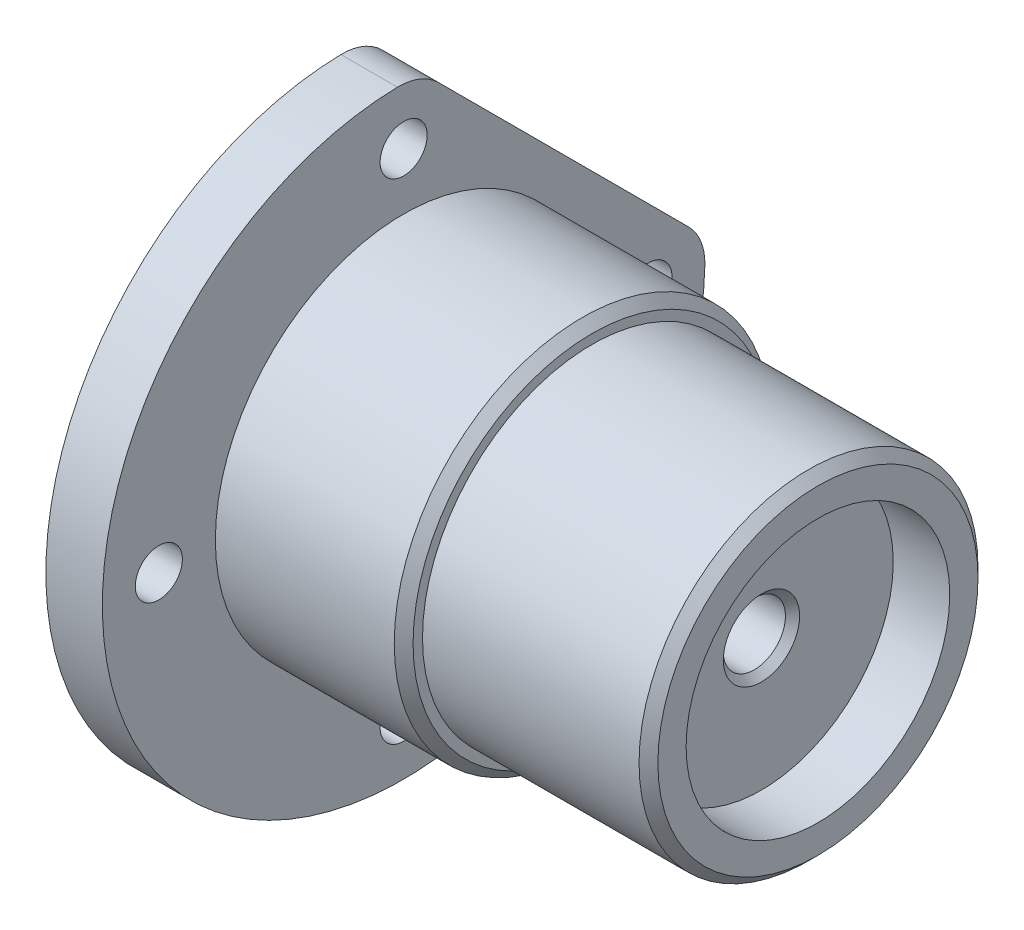
SolidWorks part; units mm, degrees
material "6061 合金"
ref_plane "前视基准面" through (0, 0, 0) normal (0, 0, 1) x (1, 0, 0)
ref_plane "上视基准面" through (0, 0, 0) normal (0, 1, 0) x (1, 0, 0)
ref_plane "右视基准面" through (0, 0, 0) normal (1, 0, 0) x (0, 0, -1)
other "Configuration Table"
sketch "草图1" plane through (0, 0, 0) normal (0, 1, 0) x (1, 0, 0)
  line L0 (-407.8675, 0) -> (19985.5084, 0) construction
  line L1 (0, 7) -> (0, 16)
  line L2 (0, 16) -> (3, 16)
  line L3 (3, 16) -> (3, 10)
  line L4 (3, 10) -> (13, 10)
  line L5 (13, 10) -> (13, 9)
  line L6 (13, 9) -> (25, 9)
  line L7 (25, 9) -> (25, 7)
  line L8 (25, 7) -> (22, 7)
  line L9 (22, 7) -> (22, 0)
  line L10 (22, 0) -> (19, 0)
  line L11 (19, 0) -> (19, 7)
  line L12 (19, 7) -> (0, 7)
  dimension "D1" = 10
  dimension "D2" = 32
  dimension "D3" = 3
  dimension "D4" = 25
  dimension "D5" = 3
  dimension "D6" = 14
  dimension "D7" = 18
  dimension "D8" = 20
  dimension "D9" = 3
revolve "旋转1" add sketch "草图1" angle 360 about L0
sketch "草图2" plane through (3, 0, 0) normal (1, 0, 0) x (0, 0, -1)
  circle A0 centre (0, 0) radius 13 construction
  circle A1 centre (0, 13) radius 1.25
  circle A2 centre (13, 0) radius 1.25
  circle A3 centre (0, -13) radius 1.25
  circle A4 centre (-13, 0) radius 1.25
  point P14 (0, 0)
  dimension "D1" = 26
  dimension "D2" = 2.5
  dimension "D3" = 4
extrude "切除-拉伸1" cut sketch "草图2" against normal through all
sketch "草图3" plane through (22, 0, 0) normal (1, 0, 0) x (0, 0, -1)
  point P0 (0, 0)
hole_wizard "M4 螺纹孔1" positions "草图3" profile "草图4" tap size "M4" standard "GB" end condition through all
sketch "草图4" plane through (22, 0, 0) normal (0, 1, 0) x (0, 0, -1)
  line L0 (0, 0) -> (0, 22)
  line L1 (0, 22) -> (1.65, 22)
  line L2 (1.65, 22) -> (1.65, 0.375)
  line L3 (1.65, 0.375) -> (2.025, 0)
  line L5 (2.025, 0) -> (0, 0)
  line L6 (-1.65, 0.375) -> (-2.025, 0) construction
  line L11 (0, -6.35) -> (0, 107.95) construction
  dimension "通孔螺纹孔钻头直径" = 3.3
  dimension "通孔螺纹孔钻头深度" = 22
  dimension "近端锥形沉头孔直径" = 4.05
  dimension "近端锥形沉头孔角度" = 90
cosmetic thread "孔螺纹线1" parameters "D2"=4
chamfer "倒角1" distance 0.5 angle 45 2 edges at (13, 0, 10) (25, 0, 9)
chamfer "倒角2" distance 1 angle 45 1 edges at (0, 0, 7)
sketch "草图5" plane through (3, 0, 0) normal (1, 0, 0) x (0, 0, -1)
  line L0 (1.002, 15.9686) -> (15.9686, 1.002)
  line L1 (0, 13) -> (13, 0) construction
  circle A0 centre (0, 0) radius 16 construction
  circle A2 centre (0, 0) radius 16
  arc A3 (15.9686, 1.002) -> (1.002, 15.9686) centre (0, 0) ccw
  dimension "D1" = 12
  dimension "D2" = 0
extrude "切除-拉伸2" cut sketch "草图5" against normal blind 10
fillet "圆角1" radius 3 2 edges at (1.5, 15.9686, -1.002) (1.5, 1.002, -15.9686)
hole_wizard "M3 螺纹孔1" positions "3D草图1" profile "草图6" tap size "M3" standard "GB" end condition through all
sketch3d "3D草图1"
  line L0 (0, 13, 0) -> (3, 13, 0) construction
  line L1 (0, 0, 13) -> (3, 0, 13) construction
  line L2 (0, -13, 0) -> (3, -13, 0) construction
  line L3 (0, 0, -13) -> (3, 0, -13) construction
  point P0 (3, 13, 0)
  point P4 (3, 0, 13)
  point P8 (3, -13, 0)
  point P12 (3, 0, -13)
sketch "草图6" plane through (3, 13, 0) normal (0, 1, 0) x (0, 0, -1)
  line L0 (0, 0) -> (0, 3)
  line L1 (0, 3) -> (1.25, 3)
  line L2 (1.25, 3) -> (1.25, 0)
  line L5 (1.25, 0) -> (0, 0)
  line L11 (0, -6.35) -> (0, 107.95) construction
  dimension "通孔螺纹孔钻头直径" = 2.5
  dimension "通孔螺纹孔钻头深度" = 3
cosmetic thread "孔螺纹线2" parameters "D2"=3
cosmetic thread "孔螺纹线3" parameters "D2"=3
cosmetic thread "孔螺纹线4" parameters "D2"=3
cosmetic thread "孔螺纹线5" parameters "D2"=3
